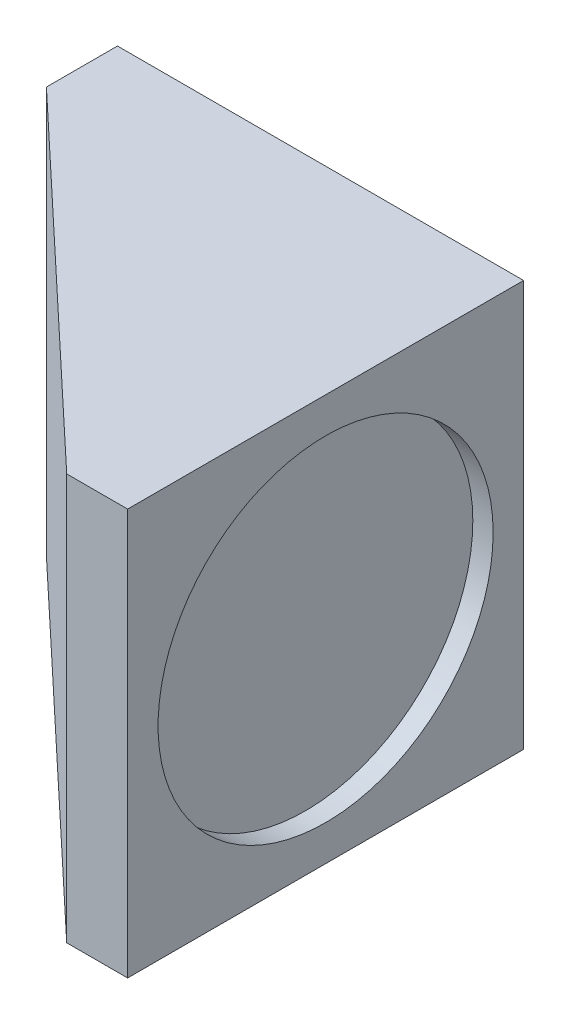
from build123d import *

# Parameters (mm, degrees)
EXTRUDE_1_DEPTH     = 40
SKETCH_2_R          = 16.5
CUT_EXTRUDE_1_DEPTH = 2


with BuildPart() as part:
    # 草图1 → 凸台-拉伸1 (new body)
    with BuildSketch(Plane(origin=(0, 0, 0), x_dir=(1, 0, 0), z_dir=(0, 1, 0))):
        Polygon((0, 0), (40, 0), (40, -39), (34, -39), (0, -7), align=None)
    extrude(amount=EXTRUDE_1_DEPTH)

    # 草图2 → 切除-拉伸1 (cut)
    with BuildSketch(Plane(origin=(40, 0, 0), x_dir=(0, 0, -1), z_dir=(1, 0, 0))):
        with Locations((-19.5, 20)):
            Circle(SKETCH_2_R)
    extrude(amount=-CUT_EXTRUDE_1_DEPTH, mode=Mode.SUBTRACT)


solid = part.part
